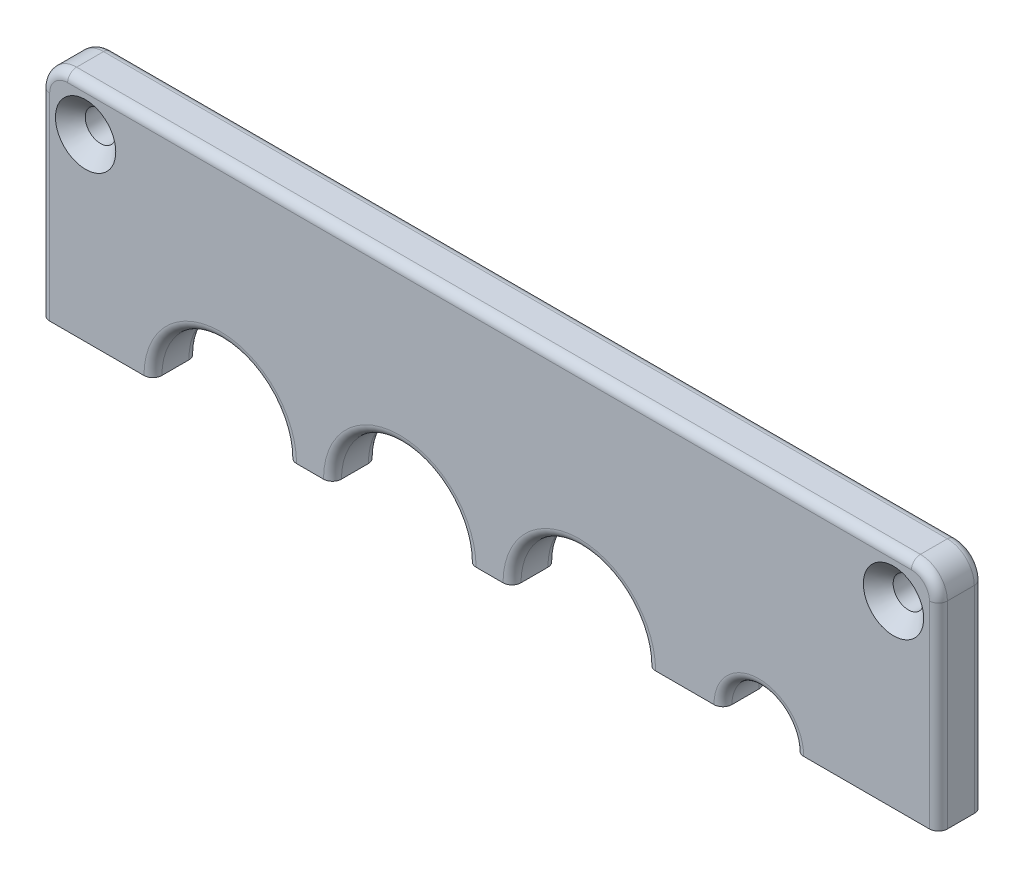
SolidWorks part; units mm, degrees
ref_plane "前视" through (0, 0, 0) normal (0, 0, 1) x (1, 0, 0)
ref_plane "上视" through (0, 0, 0) normal (0, 1, 0) x (1, 0, 0)
ref_plane "右视" through (0, 0, 0) normal (1, 0, 0) x (0, 0, -1)
sketch "草图1" plane through (0, 0, 0) normal (0, 0, 1) x (1, 0, 0)
  line L1 (0, 0) -> (100, 0)
  line L2 (0, 0) -> (0, 25)
  line L3 (0, 25) -> (100, 25)
  line L4 (100, 0) -> (100, 25)
  dimension "D1" = 25
  dimension "D2" = 100
extrude "凸台-拉伸1" add sketch "草图1" along normal blind 5
sketch "草图2" plane through (0, 0, 5) normal (0, 0, 1) x (1, 0, 0)
  line L0 (0, 0) -> (100, 0) construction
  line L1 (50, 25) -> (50, -16.1955) construction
  line L2 (100, 25) -> (0, 25) construction
  circle A0 centre (20, 0) radius 7.5
  circle A1 centre (40, 0) radius 7.5
  circle A2 centre (60, 0) radius 7.5
  circle A3 centre (80, 0) radius 4
  dimension "D1" = 8
  dimension "D3" = 15
  dimension "D4" = 15
  dimension "D2" = 20
  dimension "D5" = 60
extrude "切除-拉伸1" cut sketch "草图2" against normal through all
hole_wizard "M3 六角凹锥坑螺钉的锥形沉头孔1" positions "草图4" profile "草图3" countersink size "M3" standard "Iso" end condition through all
sketch "草图4" plane through (0, 0, 5) normal (0, 0, 1) x (1, 0, 0)
  line L0 (100, 25) -> (0, 25) construction
  line L1 (0, 25) -> (0, 0) construction
  line L2 (100, 0) -> (100, 25) construction
  point P0 (5, 20)
  point P2 (95, 20)
  dimension "D1" = 5
  dimension "D2" = 5
  dimension "D3" = 5
  dimension "D4" = 5
sketch "草图3" plane through (5, 20, 5) normal (1, 0, 0) x (0, -1, 0)
  line L0 (0, 0) -> (0, 5)
  line L1 (0, 5) -> (1.7, 5)
  line L2 (1.7, 5) -> (1.7, 1.66)
  line L3 (1.7, 1.66) -> (3.36, 0)
  line L5 (3.36, 0) -> (0, 0)
  line L6 (-1.7, 1.66) -> (-3.36, 0) construction
  line L11 (0, -6.35) -> (0, 107.95) construction
  dimension "通孔孔直径" = 3.4
  dimension "通孔孔深度" = 5
  dimension "近端锥形沉头孔直径" = 6.72
  dimension "近端锥形沉头孔角度" = 90
fillet "圆角1" radius 3 2 edges at (100, 25, 2.5) (0, 25, 2.5)
fillet "圆角2" radius 1 18 edges at (0, 11, 5) (0.8787, 24.1213, 5) (50, 25, 5) (99.1213, 24.1213, 5) (100, 11, 5) (80, 4, 0) (20, 7.5, 0) (40, 7.5, 0) (60, 7.5, 0) (80, 4, 5) (60, 7.5, 5) (40, 7.5, 5) (20, 7.5, 5) (0, 11, 0) (0.8787, 24.1213, 0) (50, 25, 0) (100, 11, 0) (99.1213, 24.1213, 0)
